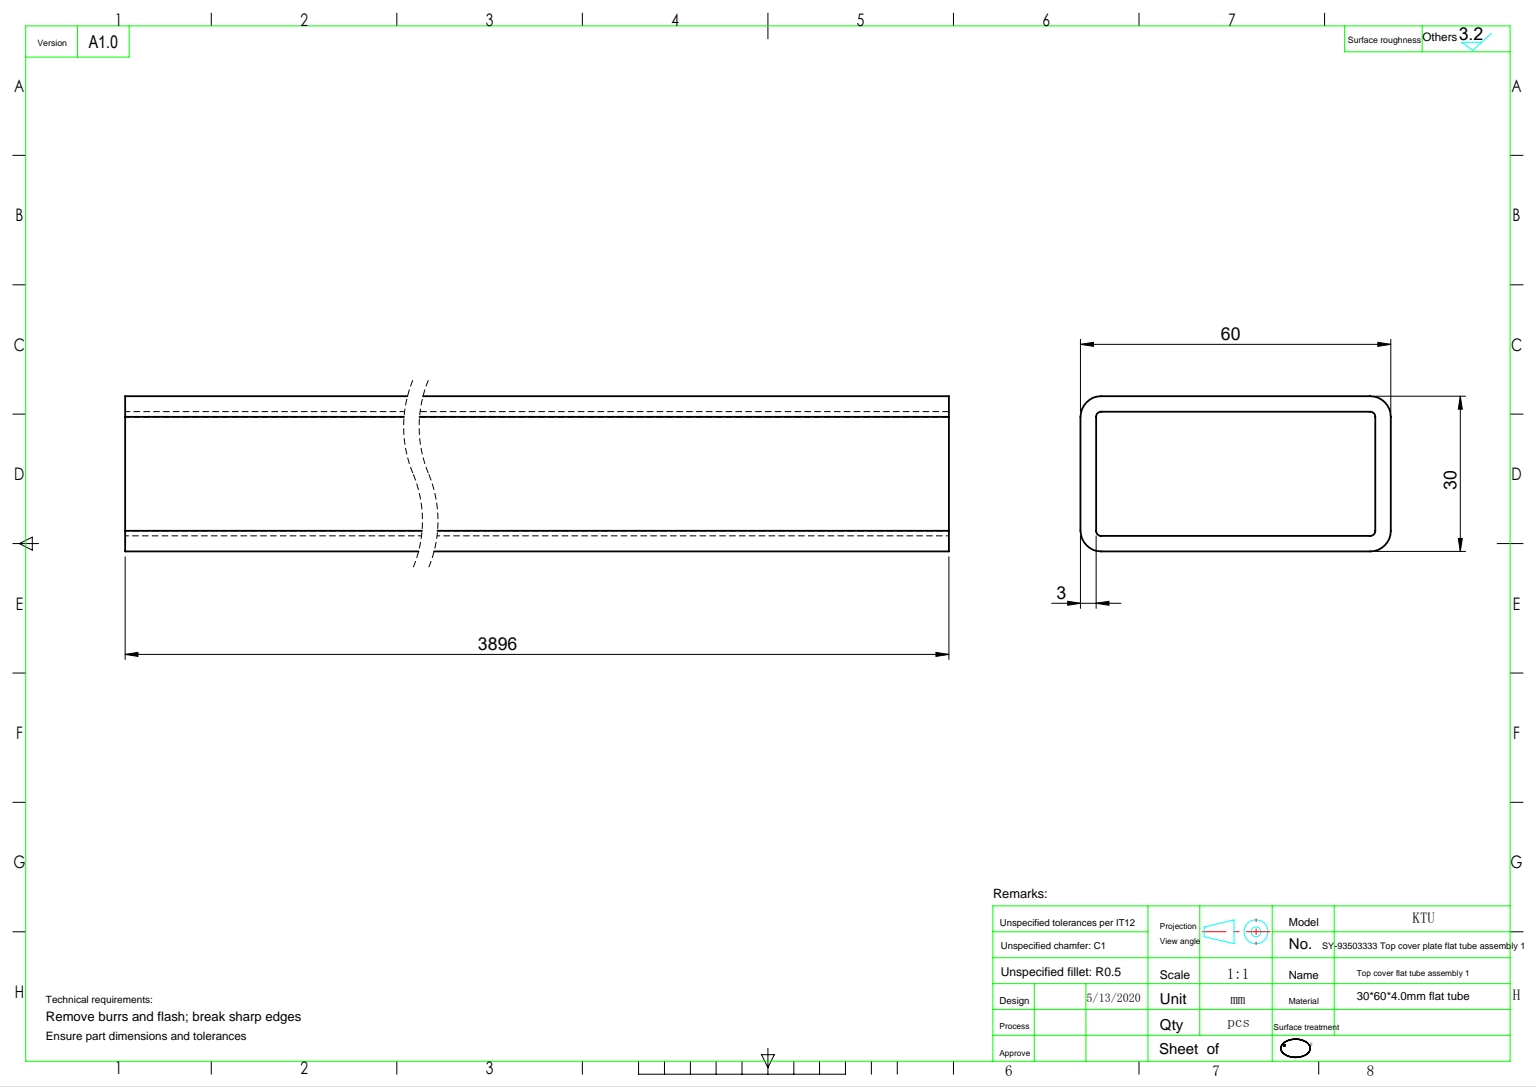
from build123d import *

# Parameters (mm, degrees)
EXTRUDE_1_DEPTH = 1948


with BuildPart() as part:
    # 草图1 → 拉伸-薄壁1 (new, symmetric)
    with BuildSketch(Plane.XY):
        with BuildLine():
            Line((-26, 15), (26, 15))
            ThreePointArc((26, 15), (28.828427125, 13.828427125), (30, 11))
            Line((30, 11), (30, -11))
            ThreePointArc((30, -11), (28.828427125, -13.828427125), (26, -15))
            Line((26, -15), (-26, -15))
            ThreePointArc((-26, -15), (-28.828427125, -13.828427125), (-30, -11))
            Line((-30, -11), (-30, 11))
            ThreePointArc((-30, 11), (-28.828427125, 13.828427125), (-26, 15))
        make_face()
        with BuildLine():
            Line((-26, 12), (26, 12))
            ThreePointArc((26, 12), (26.707106781, 11.707106781), (27, 11))
            Line((27, 11), (27, -11))
            ThreePointArc((27, -11), (26.707106781, -11.707106781), (26, -12))
            Line((26, -12), (-26, -12))
            ThreePointArc((-26, -12), (-26.707106781, -11.707106781), (-27, -11))
            Line((-27, -11), (-27, 11))
            ThreePointArc((-27, 11), (-26.707106781, 11.707106781), (-26, 12))
        make_face(mode=Mode.SUBTRACT)
    extrude(amount=EXTRUDE_1_DEPTH, both=True)


solid = part.part
